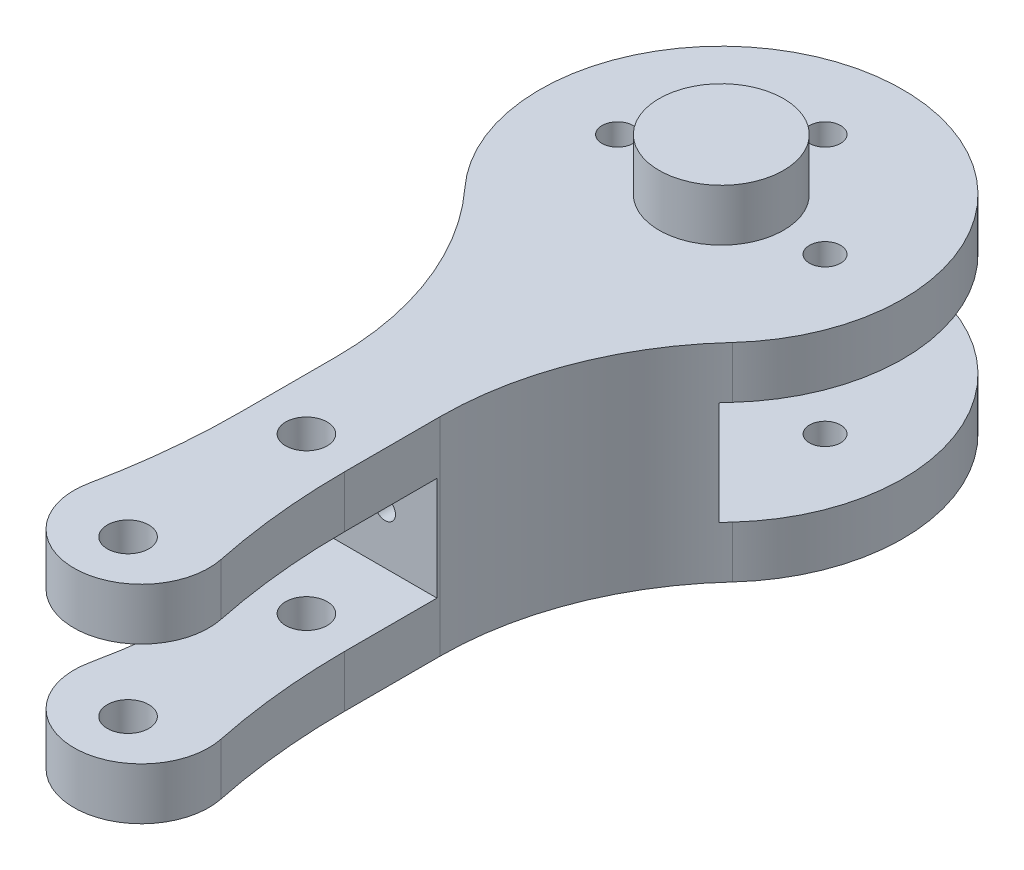
from build123d import *

# Parameters (mm, degrees)
BOSS_EXTRUDE1_DEPTH     = 20
CUT_EXTRUDE1_DEPTH      = 68.837474407
CUT_EXTRUDE1_DEPTH_BACK = 68.837474407
SKETCH2_R               = 2
SKETCH3_R               = 2
CUT_EXTRUDE2_DEPTH      = 68.837474407
SKETCH4_R               = 1.5
CUT_EXTRUDE3_DEPTH      = 68.837474407
CUT_EXTRUDE4_DEPTH      = 68.837474407
CUT_EXTRUDE4_DEPTH_BACK = 68.837474407
SKETCH5_W               = 30
SKETCH5_H               = 10
BOSS_EXTRUDE2_START     = -20
SKETCH6_R               = 6
BOSS_EXTRUDE2_DEPTH     = 5
SKETCH7_R               = 2
BOSS_EXTRUDE4_DEPTH     = 10
SKETCH8_R               = 1
CUT_EXTRUDE5_DEPTH      = 30


with BuildPart() as part:
    # Sketch1 → Boss-Extrude1 (new body)
    with BuildSketch(Plane(origin=(0, 0, 0), x_dir=(1, 0, 0), z_dir=(0, 1, 0))):
        with BuildLine():
            Line((-5, -32.113081447), (-5, -41.34652383))
            ThreePointArc((-5, -41.34652383), (-5.341807803, -48.003714064), (-6.363636364, -54.590889543))
            ThreePointArc((-6.363636364, -54.590889543), (0, -62.415326114), (6.363636364, -54.590889543))
            ThreePointArc((6.363636364, -54.590889543), (5.341807803, -48.003714064), (5, -41.34652383))
            Line((5, -41.34652383), (5, -32.113081447))
            ThreePointArc((5, -32.113081447), (7.043266511, -21.230937695), (12.894736842, -11.83113527))
            ThreePointArc((12.894736842, -11.83113527), (0, 17.5), (-12.894736842, -11.83113527))
            ThreePointArc((-12.894736842, -11.83113527), (-7.043266511, -21.230937695), (-5, -32.113081447))
        make_face()
    extrude(amount=BOSS_EXTRUDE1_DEPTH)

    # Sketch2 → Cut-Extrude1 (cut, two sides: drawn at the far end of the back side and taken through both)
    with BuildSketch(Plane(origin=(0, 20, 0), x_dir=(1, 0, 0), z_dir=(0, 1, 0)).offset(-CUT_EXTRUDE1_DEPTH_BACK)):
        with Locations(Location((0, -40, 0), (0, 0, 270))):
            Circle(SKETCH2_R)
        with Locations(Location((0, -57.194020253, 0), (0, 0, 270))):
            Circle(SKETCH2_R)
    extrude(amount=CUT_EXTRUDE1_DEPTH + CUT_EXTRUDE1_DEPTH_BACK, mode=Mode.SUBTRACT)

    # Sketch3 → Cut-Extrude2 (cut, through all)
    with BuildSketch(Plane(origin=(0, 20, 0), x_dir=(1, 0, 0), z_dir=(0, 1, 0))):
        with Locations(Location((0, 0, 0), (0, 0, 270))):
            Circle(SKETCH3_R)
    extrude(amount=-CUT_EXTRUDE2_DEPTH, mode=Mode.SUBTRACT)

    # Sketch4 → Cut-Extrude3 (cut, through all)
    with BuildSketch(Plane(origin=(0, 20, 0), x_dir=(1, 0, 0), z_dir=(0, 1, 0))):
        with Locations(Location((-10, 0, 0), (0, 0, 270))):
            Circle(SKETCH4_R)
        with Locations(Location((10, 0, 0), (0, 0, 270))):
            Circle(SKETCH4_R)
        with Locations(Location((0, 10, 0), (0, 0, 270))):
            Circle(SKETCH4_R)
    extrude(amount=-CUT_EXTRUDE3_DEPTH, mode=Mode.SUBTRACT)

    # Sketch5 → Cut-Extrude4 (cut, two sides: drawn at the far end of the back side and taken through both)
    with BuildSketch(Plane(origin=(0, 0, 0), x_dir=(0, 0, -1), z_dir=(1, 0, 0)).offset(-CUT_EXTRUDE4_DEPTH_BACK)):
        with Locations((-47.415326114, 10)):
            Rectangle(SKETCH5_W, SKETCH5_H)
        with Locations((2.5, 10)):
            Rectangle(SKETCH5_W, SKETCH5_H)
    extrude(amount=CUT_EXTRUDE4_DEPTH + CUT_EXTRUDE4_DEPTH_BACK, mode=Mode.SUBTRACT)

    # Sketch6 → Boss-Extrude2 (add)
    with BuildSketch(Plane.XZ.offset(BOSS_EXTRUDE2_START)):
        with Locations(Location((0, 0, 0), (0, 0, 270))):
            Circle(SKETCH6_R)
    extrude(amount=-BOSS_EXTRUDE2_DEPTH)

    # Sketch8 → Cut-Extrude5 (cut)
    with BuildSketch(Plane(origin=(0, 0, 12.5), x_dir=(-1, 0, 0), z_dir=(0, 0, -1))):
        with Locations((0, 9.975810979)):
            Circle(SKETCH8_R)
    extrude(amount=-CUT_EXTRUDE5_DEPTH, mode=Mode.SUBTRACT)


with BuildPart() as body_2:
    # Sketch7 → Boss-Extrude4 (new body)
    with BuildSketch(Plane(origin=(0, 5, 0), x_dir=(1, 0, 0), z_dir=(0, 1, 0))):
        with Locations(Location((0, 0, 0), (0, 0, 270))):
            Circle(SKETCH7_R)
    extrude(amount=BOSS_EXTRUDE4_DEPTH)


solid = Compound([part.part, body_2.part])
